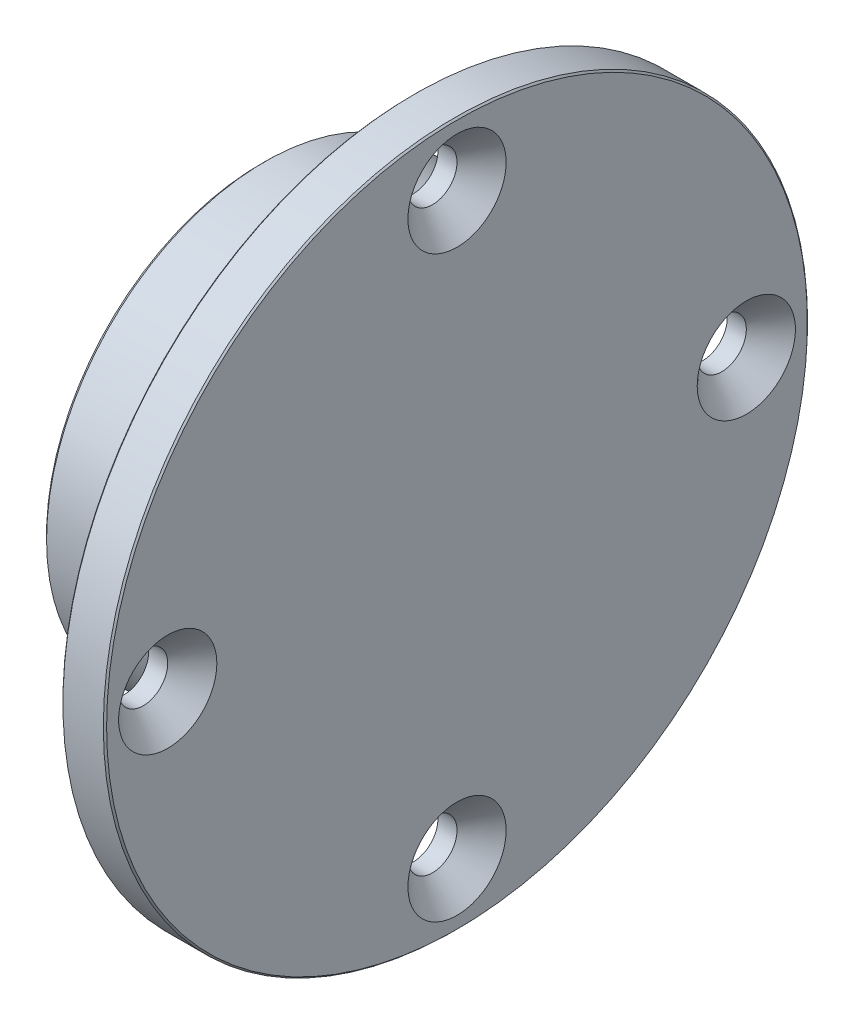
from build123d import *

# Parameters (mm, degrees)
CIRPATTERN1_COUNT  = 4
CHAMFER1_SIZE      = 0.4
CUT_EXTRUDE1_START = -10
SKETCH6_R          = 32.5
SKETCH6_R_2        = 32.25
CUT_EXTRUDE1_DEPTH = 10


with BuildPart() as part:
    # Sketch1 → Revolve1 (revolve)
    with BuildSketch(Plane.XY, mode=Mode.PRIVATE) as revolve1_sk:
        Polygon((0, 16), (1.695369244, 16), (1.695369244, 16.85), (2.995369244, 16.85), (2.995369244, 16), (13, 16), (13, 12.5), (15, 12.5), (15, 0), (18, 0), (18, 32.5), (14, 32.5), (14, 20), (0, 20), align=None)
    revolve(revolve1_sk.sketch.rotate(Axis((15, 0, 0), (1, 0, 0)), 90), axis=Axis((15, 0, 0), (1, 0, 0)))

    # Sketch2 → Cut-Revolve1 (revolve, cut)
    with BuildSketch(Plane(origin=(0, 0, 0), x_dir=(1, 0, 0), z_dir=(0, 1, 0)), mode=Mode.PRIVATE) as cut_revolve1_sk:
        Polygon((14, 26.5), (18, 26.5), (18, 31), (15.75, 28.75), (14, 28.75), align=None)
    cut_revolve1 = revolve(cut_revolve1_sk.sketch.rotate(Axis((14, 0, -26.5), (1, 0, 0)), 180), axis=Axis((14, 0, -26.5), (1, 0, 0)), mode=Mode.SUBTRACT)

    # CirPattern1: Cut-Revolve1 ×4 about axis
    cirpattern1_axis = Axis((0, 0, 0), (1, 0, 0))
    for i in range(1, CIRPATTERN1_COUNT):
        add(cut_revolve1.rotate(cirpattern1_axis, i * 360 / CIRPATTERN1_COUNT), mode=Mode.SUBTRACT)

    # Chamfer1
    chamfer1_edges = [part.edges().sort_by_distance(p)[0] for p in [
        (14, 0, -32.5),
        (18, 0, -32.5),
        (13, 0, -12.5),
        (0, 0, -16),
        (0, 0, -20),
    ]]
    chamfer(chamfer1_edges, length=CHAMFER1_SIZE)

    # Sketch6 → Cut-Extrude1 (cut)
    with BuildSketch(Plane(origin=(18, 0, 0), x_dir=(0, 0, -1), z_dir=(1, 0, 0)).offset(CUT_EXTRUDE1_START)):
        Circle(SKETCH6_R)
        Circle(SKETCH6_R_2, mode=Mode.SUBTRACT)
    extrude(amount=CUT_EXTRUDE1_DEPTH, mode=Mode.SUBTRACT)


solid = part.part
